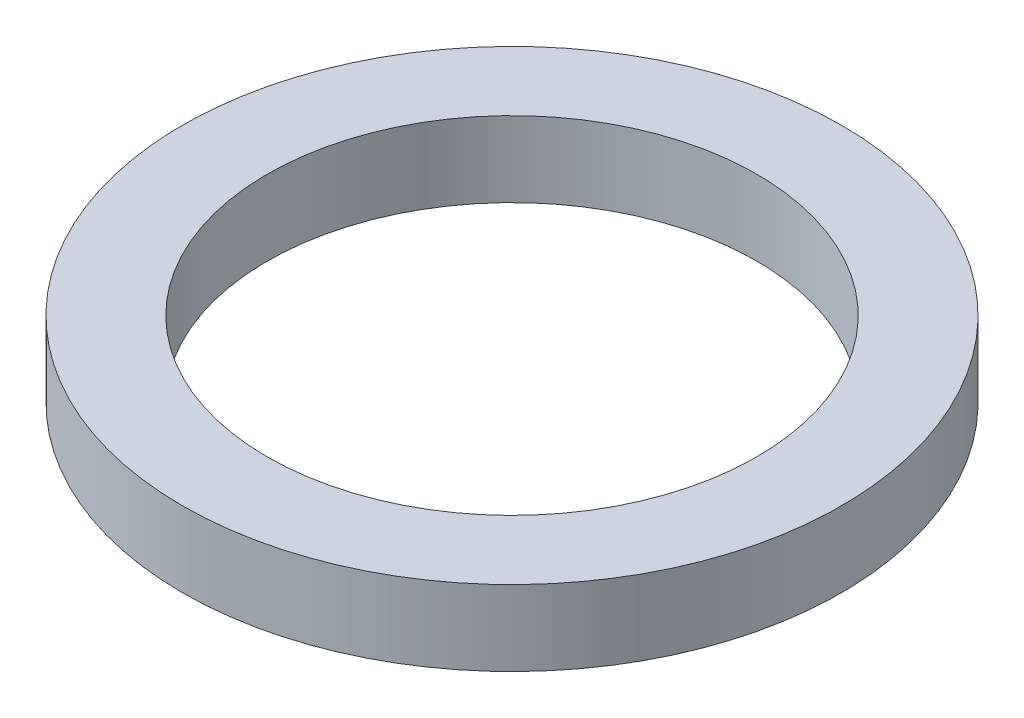
from build123d import *

# Parameters (mm, degrees)
SKETCH_1_R           = 35
SKETCH_1_R_2         = 26
BOSS_EXTRUDE_1_DEPTH = 8


with BuildPart() as part:
    # Sketch 1 → Boss-Extrude 1 (new body)
    with BuildSketch(Plane(origin=(0, 0, 0), x_dir=(1, 0, 0), z_dir=(0, 1, 0))):
        with Locations(Location((0, 0, 0), (0, 0, 270))):
            Circle(SKETCH_1_R)
        with Locations(Location((0, 0, 0), (0, 0, 270))):
            Circle(SKETCH_1_R_2, mode=Mode.SUBTRACT)
    extrude(amount=BOSS_EXTRUDE_1_DEPTH)


solid = part.part
